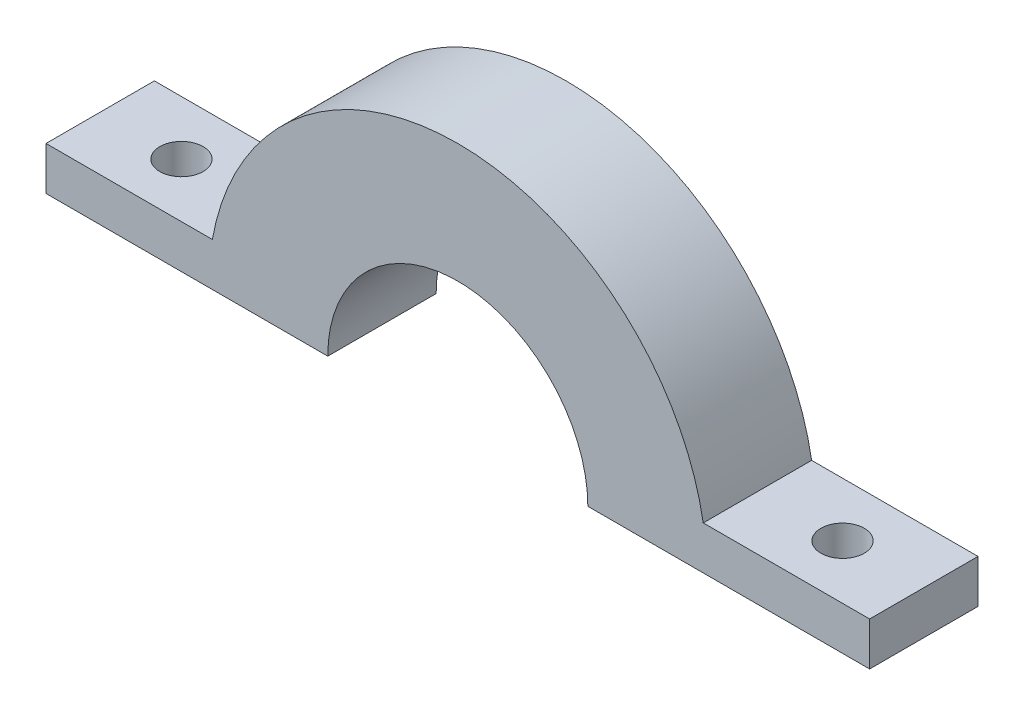
SolidWorks part; units mm, degrees
ref_plane "Front Plane" through (0, 0, 0) normal (0, 0, 1) x (1, 0, 0)
ref_plane "Top Plane" through (0, 0, 0) normal (0, 1, 0) x (1, 0, 0)
ref_plane "Right Plane" through (0, 0, 0) normal (1, 0, 0) x (0, 0, -1)
sketch "Sketch2" plane through (0, 0, 0) normal (0, 0, 1) x (1, 0, 0)
  line L0 (9.5832, 0) -> (17.0832, 0)
  line L1 (17.0832, 0) -> (17.0832, 2)
  line L2 (17.0832, 2) -> (9.4079, 2)
  line L3 (-7.9168, 0) -> (4.0832, 0)
  line L4 (-13.4168, 0) -> (-20.9168, 0)
  line L5 (-20.9168, 2) -> (-13.2416, 2)
  line L6 (-20.9168, 0) -> (-20.9168, 2)
  line L7 (-13.4168, 0) -> (-7.9168, 0)
  line L8 (4.0832, 0) -> (9.5832, 0)
  arc A1 (9.4079, 2) -> (-13.2416, 2) centre (-1.9168, 0) ccw
extrude "Boss-Extrude1" add sketch "Sketch2" along normal blind 5
sketch "Sketch3" plane through (0, 2, 0) normal (0, 1, 0) x (1, 0, 0)
  circle A0 centre (-17.1668, -2.5) radius 1
  circle A1 centre (13.3332, -2.5) radius 1
extrude "Cut-Extrude2" cut sketch "Sketch3" against normal blind 7
sketch "Sketch4" plane through (0, 0, 5) normal (0, 0, 1) x (1, 0, 0)
  line L0 (-20.9168, 0) -> (17.0832, 0) construction
  circle A0 centre (-1.9168, 0) radius 6
  dimension "D1" = 12
extrude "Cut-Extrude3" cut sketch "Sketch4" against normal through all
